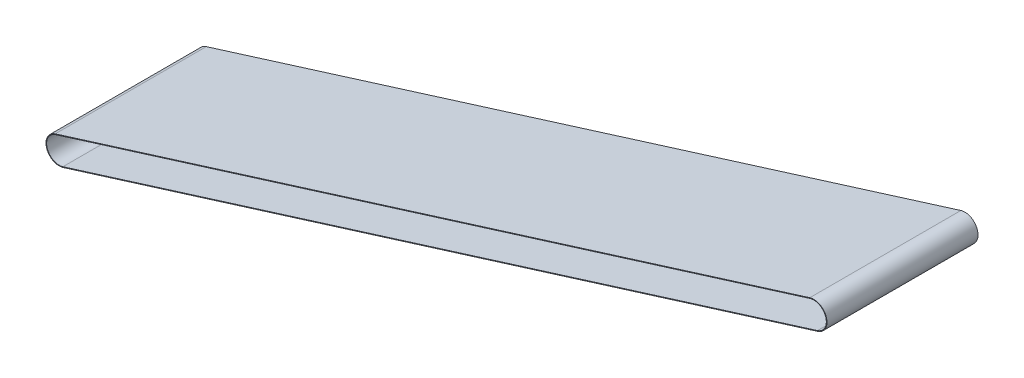
SolidWorks part; units mm, degrees
ref_plane "前视基准面" through (0, 0, 0) normal (0, 0, 1) x (1, 0, 0)
ref_plane "上视基准面" through (0, 0, 0) normal (0, 1, 0) x (1, 0, 0)
ref_plane "右视基准面" through (0, 0, 0) normal (1, 0, 0) x (0, 0, -1)
sketch "草图1" plane through (0, 0, 360) normal (0, 0, 1) x (1, 0, 0)
  line L0 (-186, 587.6) -> (3410.5, 1709.5) construction
  line L1 (-203.8674, 644.8779) -> (3392.6326, 1766.7779)
  line L2 (-168.1326, 530.3221) -> (3428.3674, 1652.2221)
  line L3 (-204.7608, 647.7418) -> (3391.7392, 1769.6418)
  line L4 (-167.2392, 527.4582) -> (3429.2608, 1649.3582)
  arc A0 (-203.8674, 644.8779) -> (-168.1326, 530.3221) centre (-186, 587.6) ccw
  arc A1 (3428.3674, 1652.2221) -> (3392.6326, 1766.7779) centre (3410.5, 1709.5) ccw
  circle A2 centre (3410.5, 1709.5) radius 60 construction
  arc A3 (3429.2608, 1649.3582) -> (3391.7392, 1769.6418) centre (3410.5, 1709.5) ccw
  arc A4 (-204.7608, 647.7418) -> (-167.2392, 527.4582) centre (-186, 587.6) ccw
  point P4 (1612.25, 1148.55)
  dimension "D1" = 3
extrude "凸台-拉伸1" add sketch "草图1" against normal up to surface (720 mm away)
